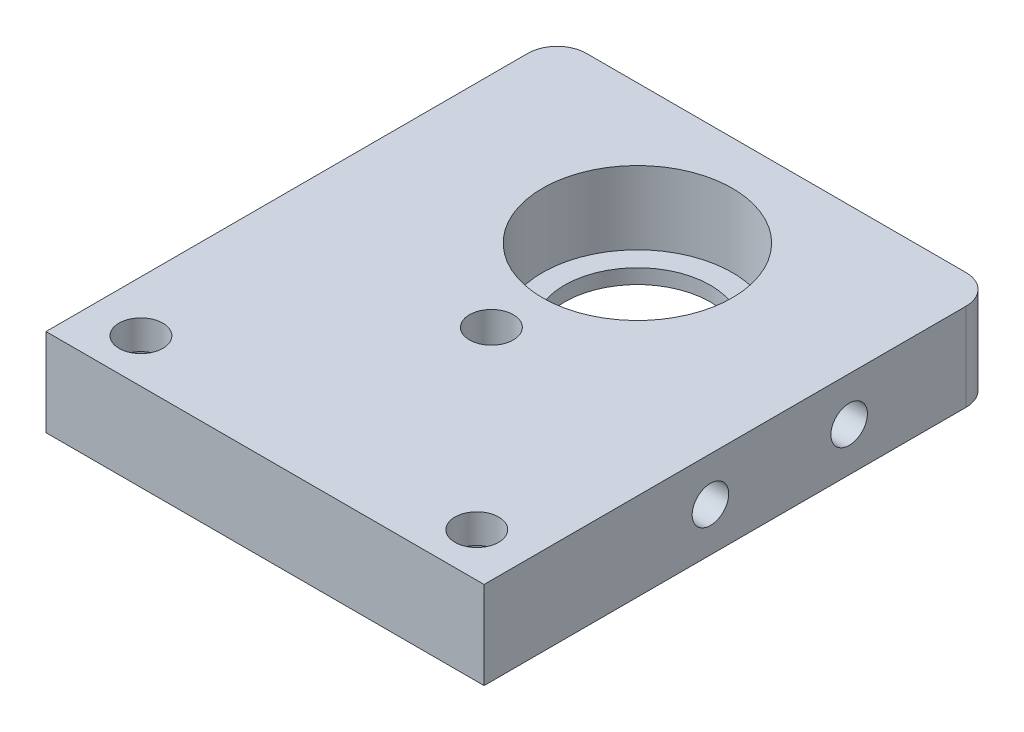
SolidWorks part; units mm, degrees
material "Q235B"
ref_plane "Front Plane" through (0, 0, 0) normal (0, 0, 1) x (1, 0, 0)
ref_plane "Top Plane" through (0, 0, 0) normal (0, 1, 0) x (1, 0, 0)
ref_plane "Right Plane" through (0, 0, 0) normal (1, 0, 0) x (0, 0, -1)
sketch "Sketch1" plane through (0, 0, 0) normal (0, 1, 0) x (1, 0, 0)
  line L1 (-13, 17.5) -> (13, 17.5)
  line L2 (-15, 15.5) -> (-15, -17.5)
  line L3 (-15, -17.5) -> (15, -17.5)
  line L4 (15, 15.5) -> (15, -17.5)
  line L5 (-15, 17.5) -> (15, -17.5) construction
  line L6 (-15, -17.5) -> (15, 17.5) construction
  circle A0 centre (0, 8) radius 5
  circle A1 centre (0, -2) radius 1.5
  arc A2 (13, 17.5) -> (15, 15.5) centre (13, 15.5) cw
  arc A3 (-13, 17.5) -> (-15, 15.5) centre (-13, 15.5) ccw
  point P0 (0, 0)
  dimension "D3" = 10
  dimension "D4" = 9.5
  dimension "D5" = 3
  dimension "D6" = 10
  dimension "D7" = 2
  dimension "D1" = 30
  dimension "D2" = 35
extrude "Boss-Extrude1" add sketch "Sketch1" along normal blind 6
sketch "Sketch3" plane through (0, 6, 0) normal (0, 1, 0) x (1, 0, 0)
  circle A0 centre (0, 8) radius 6.5
  dimension "D1" = 13
extrude "Cut-Extrude1" cut sketch "Sketch3" against normal blind 5
sketch "Sketch4" plane through (0, 6, 0) normal (0, 1, 0) x (1, 0, 0)
  line L0 (15, -17.5) -> (15, 15.5) construction
  line L1 (-15, 15.5) -> (-15, -17.5) construction
  line L2 (13, 17.5) -> (-13, 17.5) construction
  circle A0 centre (-11.5, -14.5) radius 1.5
  circle A1 centre (11.5, -14.5) radius 1.5
  dimension "D1" = 3
  dimension "D2" = 3.5
  dimension "D3" = 3.5
  dimension "D4" = 32
extrude "Cut-Extrude2" cut sketch "Sketch4" against normal through all
sketch "Sketch5" plane through (0, 0, 0) normal (0, -1, 0) x (1, 0, 0)
  circle A0 centre (11.5, 14.5) radius 2.5
  circle A1 centre (-11.5, 14.5) radius 2.5
  dimension "D1" = 5
extrude "Cut-Extrude3" cut sketch "Sketch5" against normal blind 4
sketch "Sketch6" plane through (0, 0, 0) normal (0, -1, 0) x (1, 0, 0)
  line L0 (13, -17.5) -> (-13, -17.5) construction
  line L1 (15, 17.5) -> (15, -15.5) construction
  circle A0 centre (11.5, -14) radius 1.5
  circle A1 centre (-11.5, -14) radius 1.5
  circle A2 centre (-11.5, 6) radius 1.5
  circle A3 centre (11.5, 6) radius 1.5
  dimension "D1" = 3
  dimension "D2" = 23
  dimension "D3" = 20
  dimension "D5" = 3.5
  dimension "D4" = 3.5
extrude "Cut-Extrude4" [suppressed] cut sketch "Sketch6" against normal up to next
sketch "Sketch7" [suppressed] plane through (0, 6, 0) normal (0, 1, 0) x (1, 0, 0)
  circle A0 centre (-11.5, 14) radius 2.5
  circle A1 centre (11.5, 14) radius 2.5
  circle A2 centre (11.5, -6) radius 2.5
  circle A3 centre (-11.5, -6) radius 2.5
  dimension "D1" = 5
extrude "Cut-Extrude5" [suppressed] cut sketch "Sketch7" against normal blind 4
sketch "Sketch8" plane through (15, 0, 0) normal (1, 0, 0) x (0, 0, -1)
  line L1 (17.5, 6) -> (17.5, 0) construction
  circle A0 centre (-2, 3) radius 1
  circle A1 centre (7.5, 3) radius 1
  dimension "D1" = 2
  dimension "D2" = 3
  dimension "D3" = 9.5
  dimension "D4" = 10
extrude "Cut-Extrude6" cut sketch "Sketch8" against normal blind 2
hole_wizard "M3 Tapped Hole1" positions "Sketch9" profile "Sketch10" tap size "M3" standard "GB"
sketch "Sketch9" plane through (15, 0, 0) normal (1, 0, 0) x (0, 0, -1)
  point P0 (-2, 3)
  point P3 (7.5, 3)
sketch "Sketch10" plane through (15, 3, 2) normal (0, 1, 0) x (0, 0, -1)
  line L0 (0, 0) -> (0, 8.2511)
  line L1 (0, 8.2511) -> (1.25, 7.5)
  line L2 (1.25, 7.5) -> (1.25, 0)
  line L5 (1.25, 0) -> (0, 0)
  line L10 (0, 8.2511) -> (-1.25, 7.5) construction
  line L11 (0, -6.35) -> (0, 107.95) construction
  dimension "螺纹孔钻头直径" = 2.5
  dimension "螺纹孔钻头深度" = 7.5
  dimension "导头角度" = 118
cosmetic thread "HoleThreadLine1" parameters "D1"=6, "D2"=3
cosmetic thread "HoleThreadLine2" parameters "D1"=6, "D2"=3
